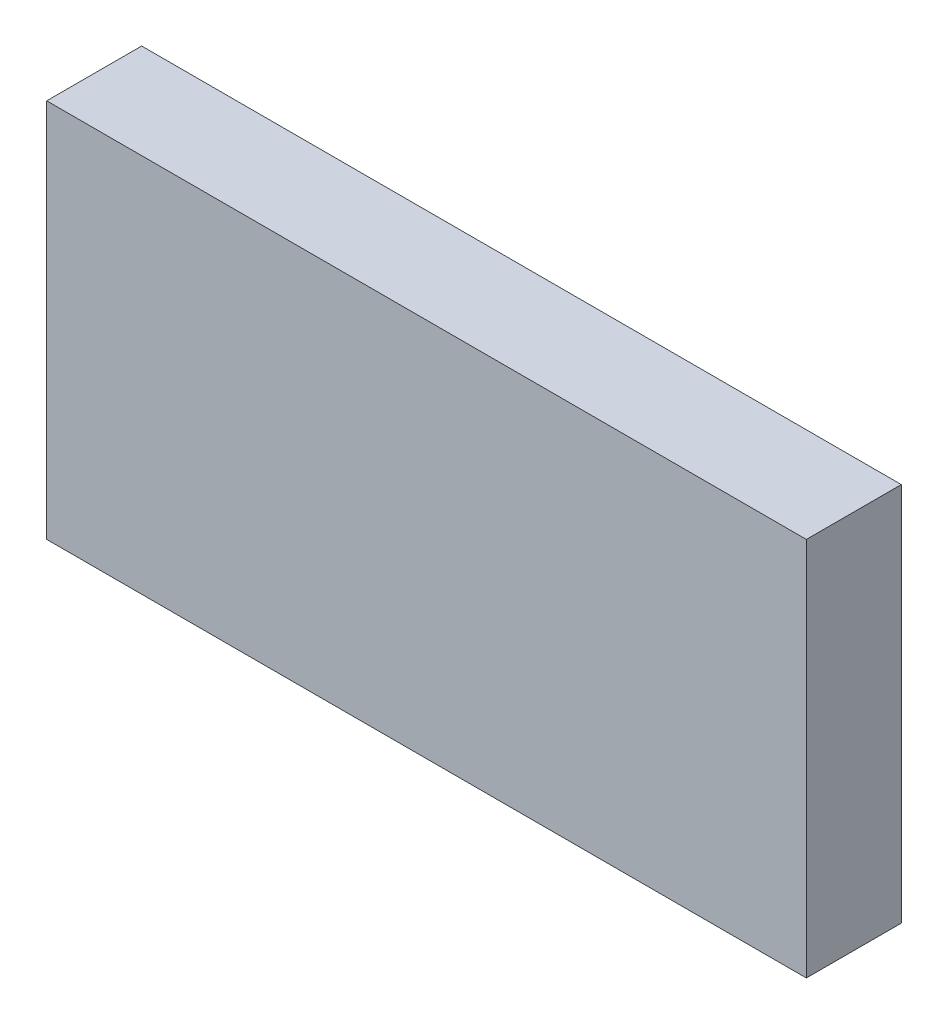
SolidWorks part; units mm, degrees
ref_plane "Front Plane" through (0, 0, 0) normal (0, 0, 1) x (1, 0, 0)
ref_plane "Top Plane" through (0, 0, 0) normal (0, 1, 0) x (1, 0, 0)
ref_plane "Right Plane" through (0, 0, 0) normal (1, 0, 0) x (0, 0, -1)
sketch "Sketch1" plane through (0, 0, 0) normal (0, 0, 1) x (1, 0, 0)
  line L1 (-31.657, 99.343) -> (208.343, 99.343)
  line L2 (-31.657, 99.343) -> (-31.657, -20.657)
  line L3 (-31.657, -20.657) -> (208.343, -20.657)
  line L4 (208.343, 99.343) -> (208.343, -20.657)
extrude "Boss-Extrude1" add sketch "Sketch1" along normal blind 30
